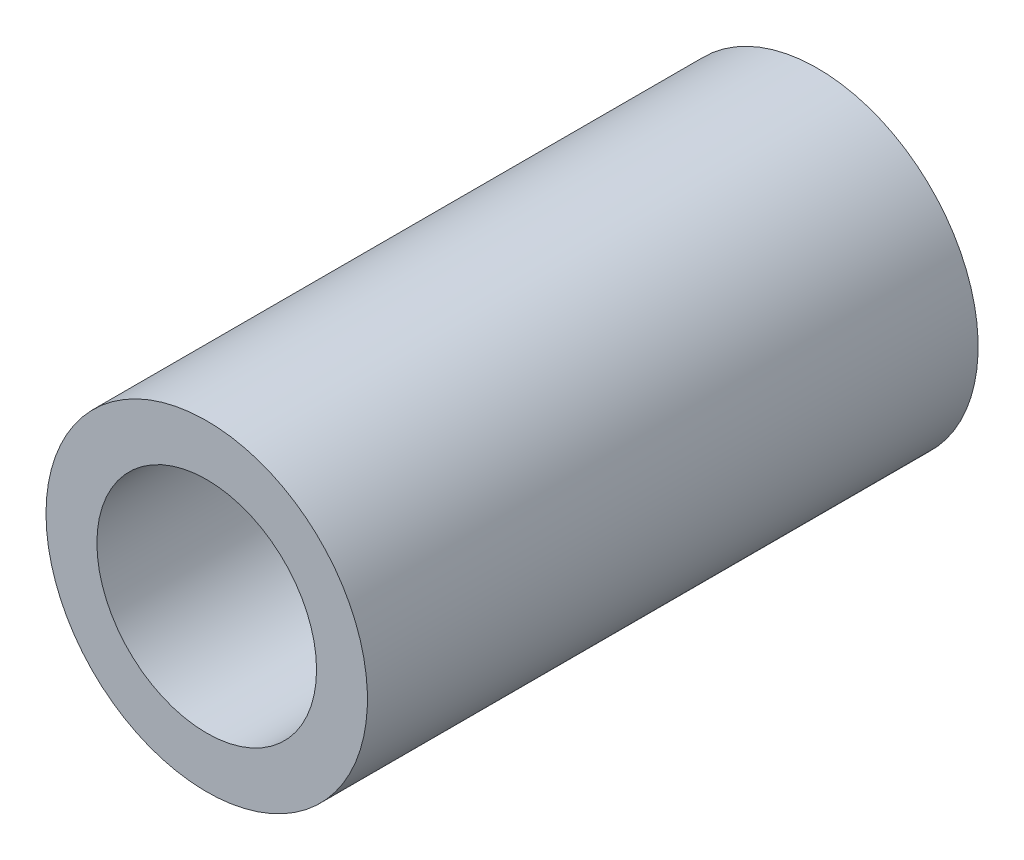
from build123d import *

# Parameters (mm, degrees)
SKETCH_1_R      = 15
SKETCH_1_R_2    = 10.25
EXTRUDE_1_DEPTH = 28.5


with BuildPart() as part:
    # 草图1 → 凸台-拉伸1 (new, symmetric)
    with BuildSketch(Plane.XY):
        with Locations(Location((0, 0, 0), (0, 0, 180))):
            Circle(SKETCH_1_R)
        with Locations(Location((0, 0, 0), (0, 0, 180))):
            Circle(SKETCH_1_R_2, mode=Mode.SUBTRACT)
    extrude(amount=EXTRUDE_1_DEPTH, both=True)


solid = part.part
